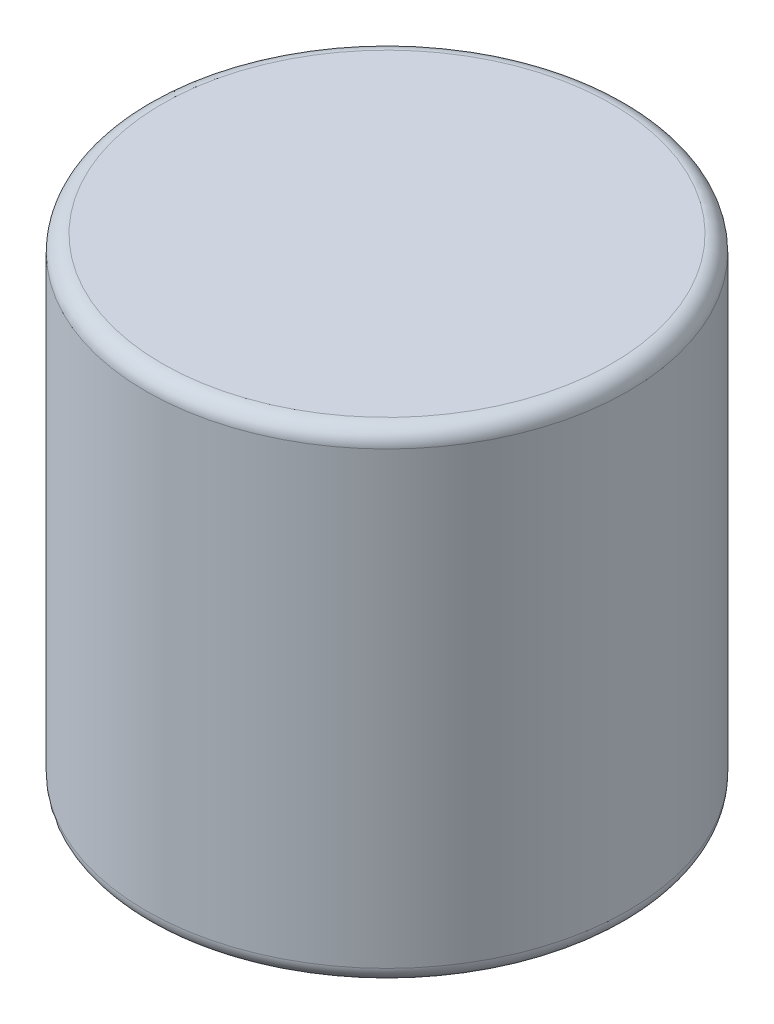
SolidWorks part; units mm, degrees
ref_plane "Front Plane" through (0, 0, 0) normal (0, 0, 1) x (1, 0, 0)
ref_plane "Top Plane" through (0, 0, 0) normal (0, 1, 0) x (1, 0, 0)
ref_plane "Right Plane" through (0, 0, 0) normal (1, 0, 0) x (0, 0, -1)
sketch "Sketch1" plane through (0, 0, 0) normal (0, 0, 1) x (1, 0, 0)
  line L0 (0, 0) -> (0, 370)
  line L1 (0, 370) -> (150, 370)
  line L2 (150, 370) -> (150, 70)
  line L3 (150, 70) -> (20, 70)
  line L4 (20, 70) -> (20, 30)
  line L5 (20, 30) -> (15, 30)
  line L6 (15, 30) -> (15, 0)
  line L7 (15, 0) -> (0, 0)
  dimension "D1" = 20
  dimension "D2" = 15
  dimension "D3" = 40
  dimension "D4" = 30
  dimension "D5" = 150
  dimension "D6" = 300
revolve "Revolve1" add sketch "Sketch1" angle 360 about L0
fillet "Fillet1" radius 10 2 edges at (0, 70, -150) (0, 370, -150)
